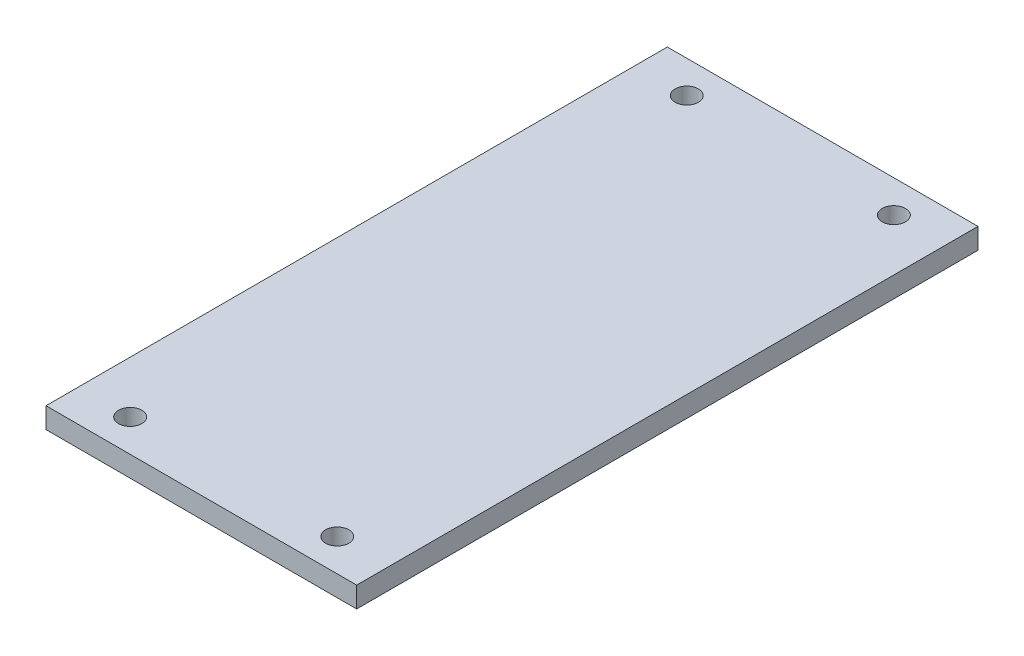
from build123d import *

# Parameters (mm, degrees)
SKETCH1_W                  = 240
SKETCH1_H                  = 480
BOSS_EXTRUDE1_DEPTH        = 16
F_18_0_18_DIAMETER_HOLE1_D = 18


with BuildPart() as part:
    # Sketch1 → Boss-Extrude1 (new body)
    with BuildSketch(Plane(origin=(0, 0, 0), x_dir=(1, 0, 0), z_dir=(0, 1, 0))):
        Rectangle(SKETCH1_W, SKETCH1_H)
    extrude(amount=BOSS_EXTRUDE1_DEPTH)

    # Ø18.0 (18) Diameter Hole1 (through all)
    with Locations(Plane(origin=(0, 16, 0), x_dir=(1, 0, 0), z_dir=(0, 1, 0))):
        with Locations((-80, -215), (80, -215), (80, 215), (-80, 215)):
            Hole(F_18_0_18_DIAMETER_HOLE1_D / 2)


solid = part.part
